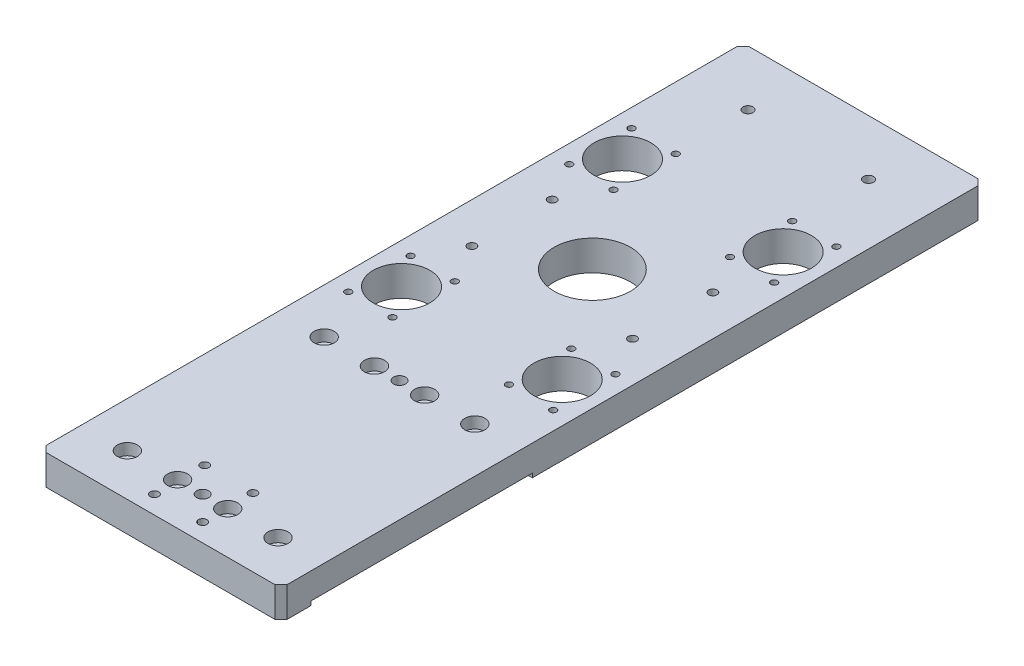
from build123d import *

# Parameters (mm, degrees)
SKETCH_1_W                = 120
SKETCH_1_H                = 350
EXTRUDE_1_DEPTH           = 15
SKETCH_3_W                = 120
SKETCH_3_H                = 110.2
CUT_EXTRUDE_1_DEPTH       = 2
HOLE_WIZARD_0_D           = 5.5
HOLE_WIZARD_0_DEPTH       = 25
HOLE_WIZARD_0_CBORE_D     = 10
HOLE_WIZARD_0_CBORE_DEPTH = 5.7
HOLE_WIZARD_0_TIP         = 1.652366702
MM_1_D                    = 6
MM_1_DEPTH                = 25
MM_1_TIP                  = 1.802581857
CHAMFER_1_SIZE            = 3
SKETCH_8_R                = 19
CUT_EXTRUDE_2_DEPTH       = 20
SKETCH_9_R                = 14.1
CUT_EXTRUDE_3_DEPTH       = 20
MM_2_D                    = 5
MM_2_DEPTH                = 20
MM_2_TIP                  = 1.502151548
HOLE_WIZARD_M5_1_D        = 4.2
HOLE_WIZARD_M5_1_DEPTH    = 20
HOLE_WIZARD_M5_1_TIP      = 1.2618073
HOLE_WIZARD_M4_1_D        = 3.3
HOLE_WIZARD_M4_1_DEPTH    = 32
HOLE_WIZARD_M4_1_TIP      = 0.991420021
HOLE_WIZARD_M5_2_D        = 4.2
HOLE_WIZARD_M5_2_DEPTH    = 20
HOLE_WIZARD_M5_2_TIP      = 1.2618073


with BuildPart() as part:
    # 草图1 → 凸台-拉伸1 (new body)
    with BuildSketch(Plane(origin=(0, 0, 0), x_dir=(1, 0, 0), z_dir=(0, 1, 0))):
        Rectangle(SKETCH_1_W, SKETCH_1_H)
    extrude(amount=EXTRUDE_1_DEPTH)

    # 草图3 → 切除-拉伸1 (cut)
    with BuildSketch(Plane.XZ):
        with Locations((0, 105)):
            Rectangle(SKETCH_3_W, SKETCH_3_H)
    extrude(amount=-CUT_EXTRUDE_1_DEPTH, mode=Mode.SUBTRACT)

    # 打孔尺寸(%根据)内六角圆柱头螺钉的类型0
    with Locations(Plane(origin=(0, 15, 0), x_dir=(1, 0, 0), z_dir=(0, 1, 0))):
        with Locations((-37.5, -154), (-12.5, -154), (12.5, -154), (37.5, -154), (-37.5, -56), (-12.5, -56), (12.5, -56), (37.5, -56)):
            CounterBoreHole(HOLE_WIZARD_0_D / 2, HOLE_WIZARD_0_CBORE_D / 2, HOLE_WIZARD_0_CBORE_DEPTH, depth=HOLE_WIZARD_0_DEPTH)
            with Locations((0, 0, -(HOLE_WIZARD_0_DEPTH + HOLE_WIZARD_0_TIP / 2))):  # 118° drill point
                Cone(0, HOLE_WIZARD_0_D / 2, HOLE_WIZARD_0_TIP, mode=Mode.SUBTRACT)

    # 大小mm 暗销孔1
    with Locations(Plane(origin=(0, 15, 0), x_dir=(1, 0, 0), z_dir=(0, 1, 0))):
        with Locations((0, -154), (0, -56)):
            Hole(MM_1_D / 2, depth=MM_1_DEPTH)
            with Locations((0, 0, -(MM_1_DEPTH + MM_1_TIP / 2))):  # 118° drill point
                Cone(0, MM_1_D / 2, MM_1_TIP, mode=Mode.SUBTRACT)

    # 倒角1
    chamfer_1_edges = [part.edges().sort_by_distance(p)[0] for p in [
        (60, 7.5, 175),
        (-60, 7.5, 175),
        (-60, 7.5, -175),
        (60, 7.5, -175),
    ]]
    chamfer(chamfer_1_edges, length=CHAMFER_1_SIZE)

    # 草图8 → 切除-拉伸2 (cut)
    with BuildSketch(Plane(origin=(0, 15, 0), x_dir=(1, 0, 0), z_dir=(0, 1, 0))):
        with Locations(Location((0, 40, 0), (0, 0, 270))):
            Circle(SKETCH_8_R)
    extrude(amount=-CUT_EXTRUDE_2_DEPTH, mode=Mode.SUBTRACT)

    # 草图9 → 切除-拉伸3 (cut)
    with BuildSketch(Plane(origin=(0, 15, 0), x_dir=(1, 0, 0), z_dir=(0, 1, 0))):
        with Locations(Location((40, -15, 0), (0, 0, 270))):
            Circle(SKETCH_9_R)
        with Locations(Location((40, 95, 0), (0, 0, 270))):
            Circle(SKETCH_9_R)
        with Locations(Location((-40, -15, 0), (0, 0, 270))):
            Circle(SKETCH_9_R)
        with Locations(Location((-40, 95, 0), (0, 0, 270))):
            Circle(SKETCH_9_R)
    extrude(amount=-CUT_EXTRUDE_3_DEPTH, mode=Mode.SUBTRACT)

    # 大小mm 暗销孔2
    with Locations(Plane(origin=(0, 15, 0), x_dir=(1, 0, 0), z_dir=(0, 1, 0))):
        with Locations((29.999999981, 147.499999979), (-30.000000019, 147.499999979)):
            Hole(MM_2_D / 2, depth=MM_2_DEPTH)
            with Locations((0, 0, -(MM_2_DEPTH + MM_2_TIP / 2))):  # 118° drill point
                Cone(0, MM_2_D / 2, MM_2_TIP, mode=Mode.SUBTRACT)

    # M5 螺纹孔1
    with Locations(Plane(origin=(0, 0, 0), x_dir=(-1, 0, 0), z_dir=(0, -1, 0))):
        with Locations((39.999999998, 19.999999998), (-40.000000002, 19.999999998), (39.999999998, 59.999999998), (-40.000000002, 59.999999998)):
            Hole(HOLE_WIZARD_M5_1_D / 2, depth=HOLE_WIZARD_M5_1_DEPTH)
            with Locations((0, 0, -(HOLE_WIZARD_M5_1_DEPTH + HOLE_WIZARD_M5_1_TIP / 2))):  # 118° drill point
                Cone(0, HOLE_WIZARD_M5_1_D / 2, HOLE_WIZARD_M5_1_TIP, mode=Mode.SUBTRACT)

    # M4 螺纹孔1
    with Locations(Plane(origin=(0, 15, 0), x_dir=(1, 0, 0), z_dir=(0, 1, 0))):
        with Locations((51, -30.5), (29, -30.5), (51, 0.5), (29, 0.5), (-51, -30.5), (-29, -30.5), (-29, 0.5), (-51, 0.5), (51, 79.5), (29, 79.5), (51, 110.5), (29, 110.5), (-29, 79.5), (-51, 79.5), (-29, 110.5), (-51, 110.5)):
            Hole(HOLE_WIZARD_M4_1_D / 2, depth=HOLE_WIZARD_M4_1_DEPTH)
            with Locations((0, 0, -(HOLE_WIZARD_M4_1_DEPTH + HOLE_WIZARD_M4_1_TIP / 2))):  # 118° drill point
                Cone(0, HOLE_WIZARD_M4_1_D / 2, HOLE_WIZARD_M4_1_TIP, mode=Mode.SUBTRACT)

    # M5 螺纹孔2
    with Locations(Plane(origin=(0, 15, 0), x_dir=(1, 0, 0), z_dir=(0, 1, 0))):
        with Locations((-11.999999999, -141.000000001), (12.000000001, -141.000000001), (-11.999999999, -166.000000001), (12.000000001, -166.000000001)):
            Hole(HOLE_WIZARD_M5_2_D / 2, depth=HOLE_WIZARD_M5_2_DEPTH)
            with Locations((0, 0, -(HOLE_WIZARD_M5_2_DEPTH + HOLE_WIZARD_M5_2_TIP / 2))):  # 118° drill point
                Cone(0, HOLE_WIZARD_M5_2_D / 2, HOLE_WIZARD_M5_2_TIP, mode=Mode.SUBTRACT)


solid = part.part
